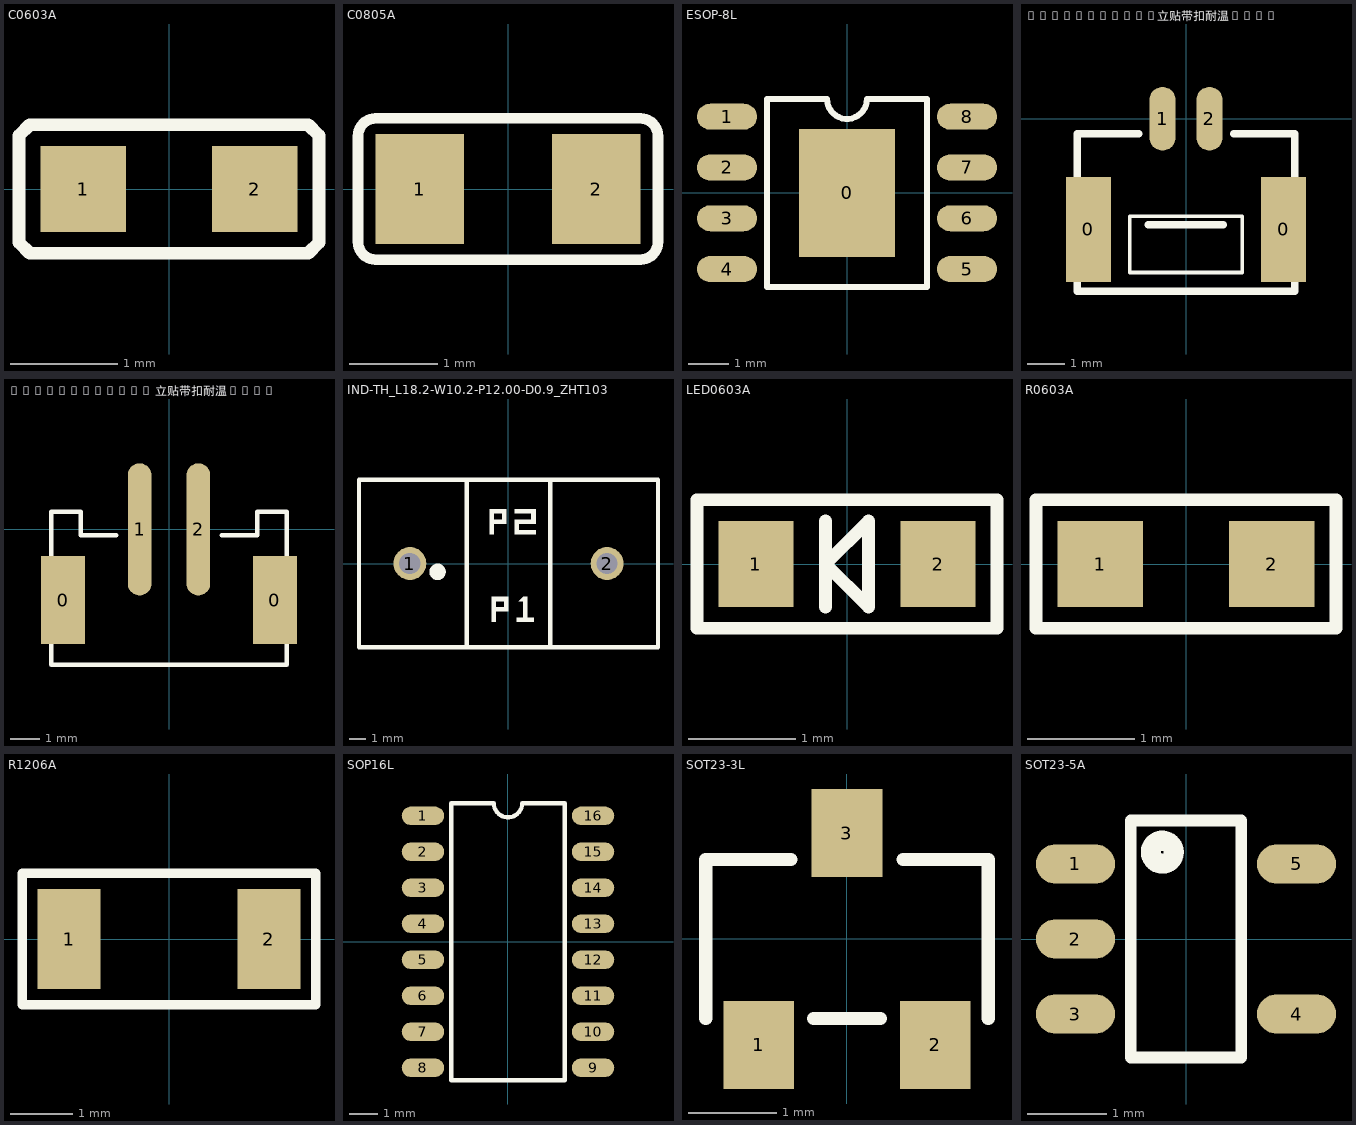
[diagram p0: the footprints below, top view; thin cyan lines are the x and y axes]
# Altium footprint library MISC84244-2.PcbLib: 12 footprints
Each footprint in its own frame and in the unit in brackets; x right, y up, seen from the top. Pads: shape width x height; smd on the part's side, far side on the other; paste and mask are expansions set on the pad; w line width, h text height; cw(c..) or ccw(c..) is an arc to the next point about the centre after c.

## C0603A [mm] "SMD capacitor"
pads (2):
  rect 0.8x0.8 smd mask+0.08: 1(-0.8,0) 2(0.8,0)
Top Overlay:
  lines w0.12: 0.551,-0.6 1.2,-0.6 ; -1.4,-0.5 -1.3,-0.6 1.3,-0.6 1.4,-0.5 1.4,0.5 1.3,0.6 -1.3,0.6 -1.4,0.5 -1.4,-0.5

## C0805A [mm] "SMD capacitor"
pads (2):
  rect 1x1.25 smd: 1(-1,0)
  rect 1x1.25 smd mask+0.102: 2(1,0)
Top Overlay:
  lines w0.12: -1.7,-0.6 ccw(c-1.5,-0.6) -1.5,-0.8 1.5,-0.8 ccw(c1.5,-0.6) 1.7,-0.6 1.7,0.6 ccw(c1.5,0.6) 1.5,0.8 -1.5,0.8 ccw(c-1.5,0.6) -1.7,0.6 -1.7,-0.6

## ESOP-8L [mm] "SMD MOS/IC"
pads (9):
  rect 2.4x3.2 smd: 0(0,0)
  oval 1.5x0.65 smd: 1(-3,1.905) 2(-3,0.635) 3(-3,-0.635) 4(-3,-1.905) 5(3,-1.905) 6(3,-0.635) 7(3,0.635) 8(3,1.905)
Top Overlay:
  lines w0.15: -2,-2.35 -2,2.35 -0.5,2.35 ccw(c0,2.35) 0.5,2.35 2,2.35 2,-2.35 -2,-2.35

## GH1.25-2PIN立贴带扣耐温260℃ [mm] "Vertical SMD, latched, rated 260℃"
pads (4):
  rect 1.2x2.8 smd: 0(-2.6,-2.95) 0(2.6,-2.95)
  oval 0.7x1.7 smd: 1(-0.625,0) 2(0.625,0)
Top Overlay:
  lines w0.1: -1.5,-4.1 -1.5,-2.6 1.5,-2.6 1.5,-4.1 -1.5,-4.1
  lines w0.2: -2.9,-0.4 -2.9,-4.6 2.9,-4.6 2.9,-0.4 1.27,-0.4 ; -2.895,-0.4 -1.265,-0.4 ; -1,-2.825 1,-2.825

## HY2.0WT-2A/P 立贴带扣耐温260℃ [mm] "Horizontal SMD connector"
pads (4):
  rect 1.5x3 smd: 0(-3.6,-2.4) 0(3.6,-2.4)
  oval 0.8x4.5 smd: 1(-1,0) 2(1,0)
Top Overlay:
  lines w0.15: -1.8,-0.2 -3,-0.2 -3,0.6 -4,0.6 -4,-4.6 4,-4.6 4,0.6 3,0.6 3,-0.2 1.8,-0.2

## IND-TH_L18.2-W10.2-P12.00-D0.9_ZHT103 [mm]
pads (2):
  round 2 hole 1.3: 1(-6,0) 2(6,0)
Top Overlay:
  circle w0.5: c-4.318,-0.508 r0.25
  region: 0.635,-2.286 0.889,-2.032 1.143,-2.032 1.143,-3.302 1.524,-3.302 1.524,-3.556 0.508,-3.556 0.508,-3.302 0.889,-3.302 0.889,-2.286
  region: -0.762,-2.032 0,-2.032 0,-2.921 -0.762,-2.921 -0.762,-2.667 -0.254,-2.667 -0.254,-2.286 -0.762,-2.286
  region: -1.016,-2.032 -1.016,-3.556 -0.762,-3.556 -0.762,-2.032
  region: -0.889,3.302 -0.127,3.302 -0.127,2.413 -0.889,2.413 -0.889,2.667 -0.381,2.667 -0.381,3.048 -0.889,3.048
  region: -1.143,3.302 -1.143,1.778 -0.889,1.778 -0.889,3.302
  region: 0.381,3.302 1.651,3.302 1.651,3.048 1.651,2.413 0.635,2.413 0.635,2.032 1.651,2.032 1.651,1.778 0.381,1.778 0.381,2.667 1.397,2.667 1.397,3.048 0.381,3.048
  lines w0.254: -9.1,-5.1 9.1,-5.1 9.1,5.1 -9.1,5.1 -9.1,-5.1 ; -2.54,-5.08 2.54,-5.08 2.54,5.08 -2.54,5.08 -2.54,-5.08
Mechanical 8:
  region: -9.04,-5.1 -9.04,-5.125 -9.075,-5.16 -9.125,-5.16 -9.16,-5.125 -9.16,-5.1 -9.16,-5.075 -9.125,-5.04 -9.075,-5.04 -9.04,-5.075 -9.04,-5.1

## LED0603A [mm] "SMD LED"
pads (2):
  rect 0.7x0.8 smd: 1(-0.85,0) 2(0.85,0)
Top Overlay:
  lines w0.12: -0.2,-0.4 -0.2,0.4 ; -1.4,-0.6 1.4,-0.6 1.4,0.6 -1.4,0.6 -1.4,-0.6 ; -0.2,0 0.2,-0.4 0.2,0.4 -0.2,0

## R0603A [mm] "SMD resistor"
height 0.5
pads (2):
  rect 0.8x0.8 smd mask+0.08: 1(-0.8,0) 2(0.8,0)
Top Overlay:
  lines w0.12: -1.4,-0.6 1.4,-0.6 1.4,0.6 -1.4,0.6 -1.4,-0.6

## R1206A [mm] "SMD resistor"
pads (2):
  rect 1x1.6 smd: 1(-1.6,0) 2(1.6,0)
Top Overlay:
  lines w0.15: -2.35,-1.05 -2.35,1.05 2.35,1.05 2.35,-1.05 -2.35,-1.05

## SOP16L [mm]
pads (16):
  oval 1.5x0.65 smd: 1(-3,4.445) 2(-3,3.175) 3(-3,1.905) 4(-3,0.635) 5(-3,-0.635) 6(-3,-1.905) 7(-3,-3.175) 8(-3,-4.445) 9(3,-4.445) 10(3,-3.175) 11(3,-1.905) 12(3,-0.635) 13(3,0.635) 14(3,1.905) 15(3,3.175) 16(3,4.445)
Top Overlay:
  lines w0.15: -2,-4.89 -2,4.89 -0.5,4.89 ccw(c0,4.89) 0.5,4.89 2,4.89 2,-4.89 -2,-4.89

## SOT23-3L [mm] "SMD MOS"
pads (3):
  rect 0.8x1 smd: 1(-1,-1.2) 2(1,-1.2) 3(0,1.2)
Top Overlay:
  lines w0.15: -1.6,-0.9 -1.6,0.9 -0.635,0.9 ; -0.381,-0.9 0.381,-0.9 ; 0.635,0.9 1.6,0.9 1.6,-0.9

## SOT23-5A [mm] "SMD IC"
pads (5):
  oval 1x0.5 smd mask+0.05: 1(-1.4,0.95) 2(-1.4,0) 3(-1.4,-0.95) 4(1.4,-0.95) 5(1.4,0.95)
Top Overlay:
  circle w0.254: c-0.3,1.1 r0.146
  lines w0.15: -0.7,-1.5 -0.7,1.5 0.7,1.5 0.7,-1.5 -0.7,-1.5